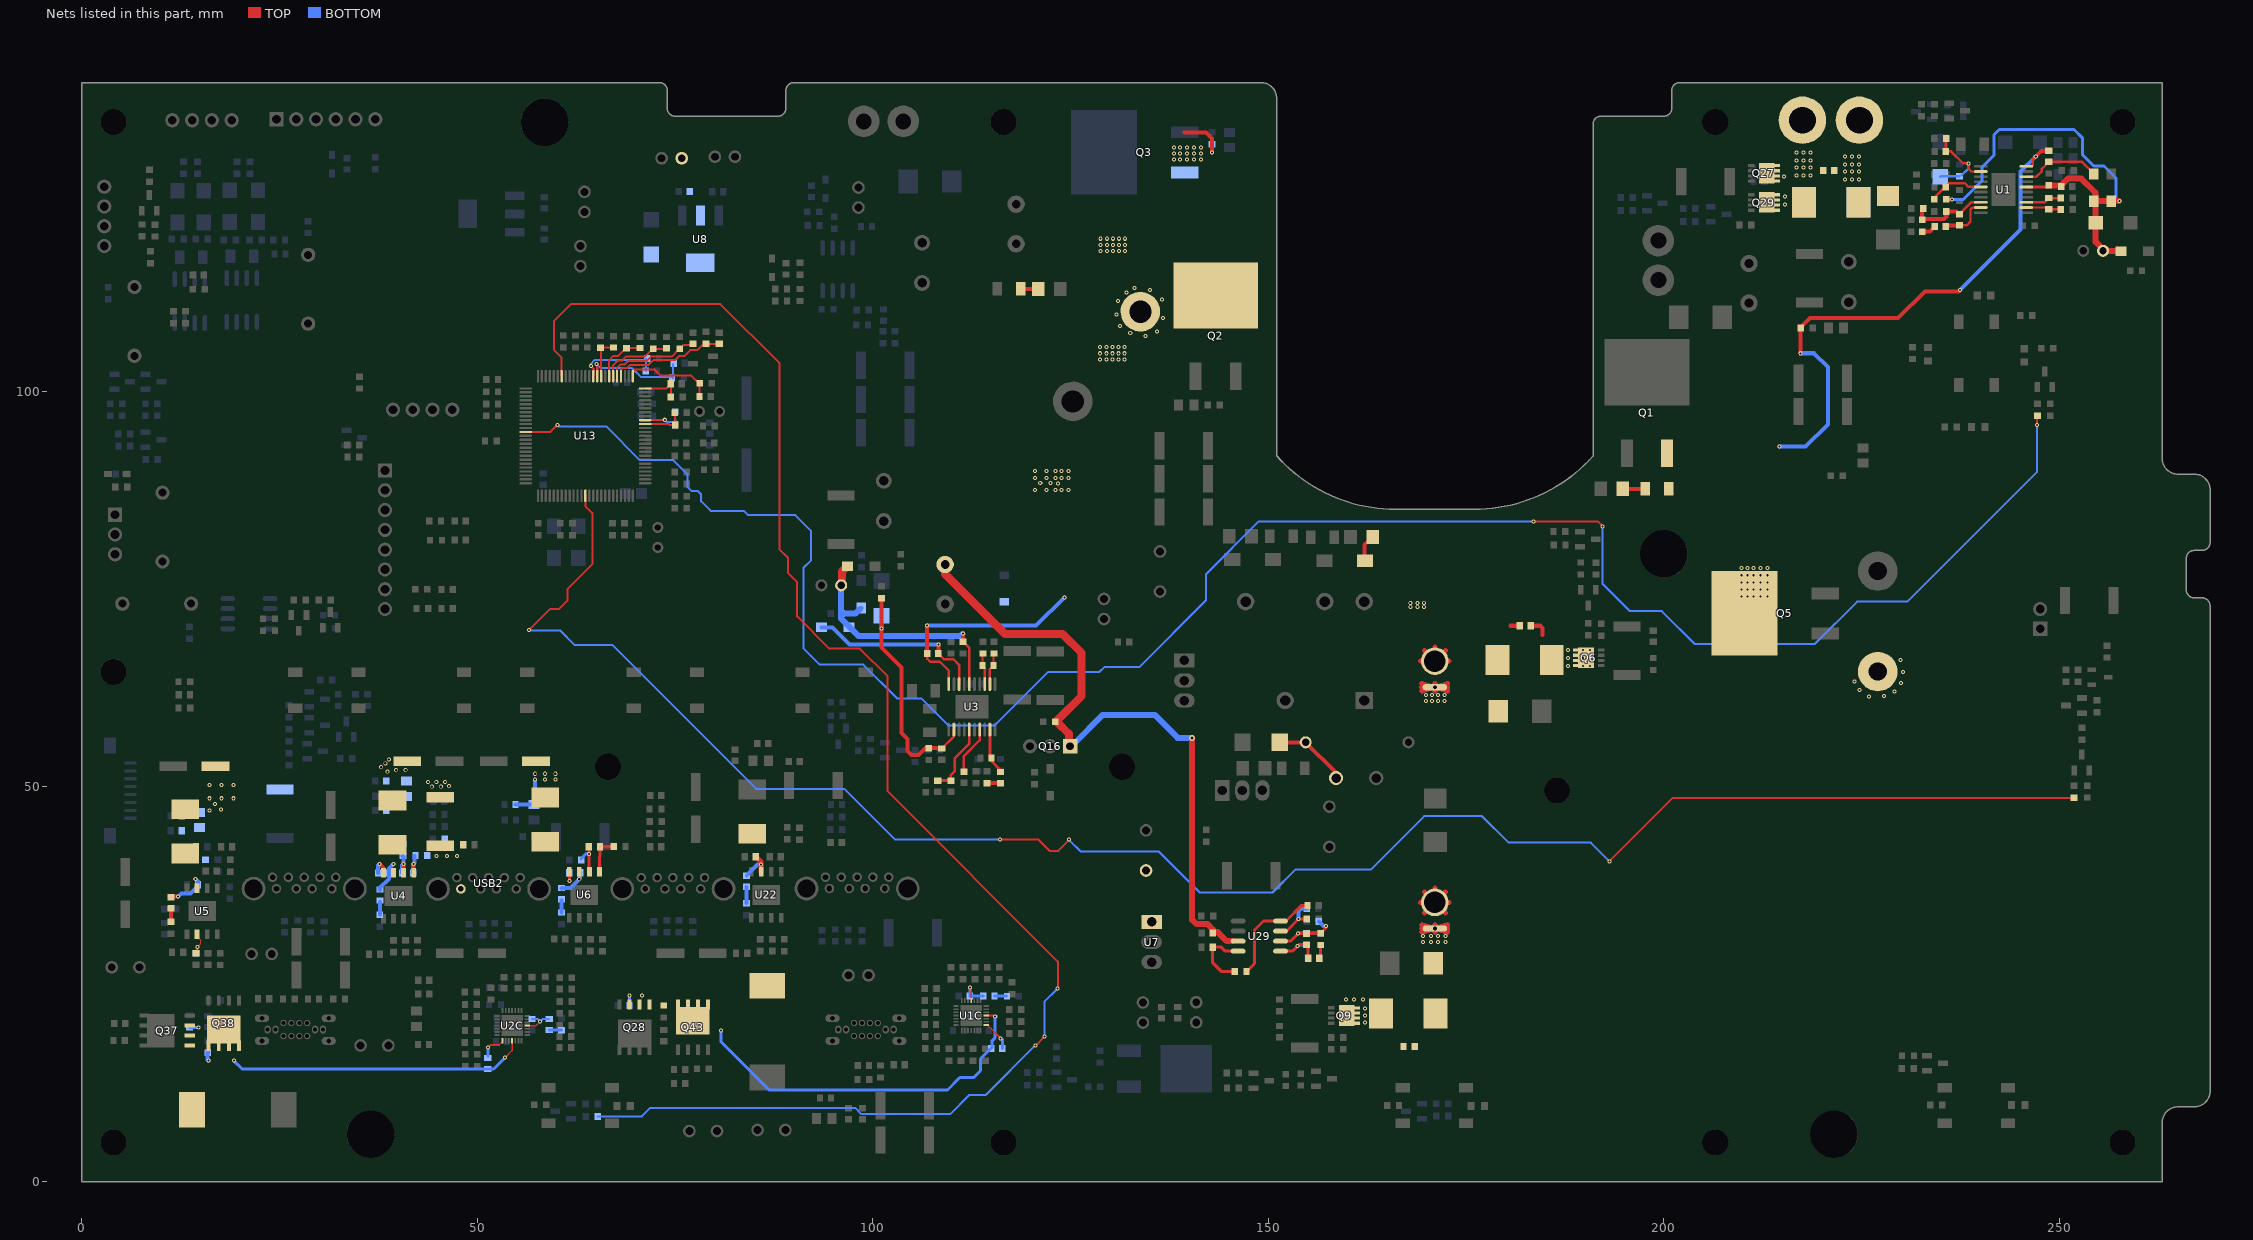
[diagram p0: the nets of this part, all layers, seen from the top]
# Altium PCB MISC84402.PcbDoc (part 6 of 12)
Units mm, origin at the board's own origin, x right, y up, seen from the top; angles counter-clockwise.
Board outline 269.06 x 139 mm, 4 copper layers (TOP, GND02, PWR03, BOTTOM), stack 0.732 mm thick; 694 components, 428 nets, 1859 pads, 1384 vias.

## Via types
v1: diameter 0.508, hole 0.254, TOP to BOTTOM, tented both sides, 1015 vias
v2: diameter 0.508, hole 0.254, TOP to BOTTOM, 243 vias
v3: diameter 0.508, hole 0.305, TOP to BOTTOM, 60 vias
v4: diameter 0.61, hole 0.305, TOP to BOTTOM, 55 vias
v5: diameter 0.61, hole 0.305, TOP to BOTTOM, tented both sides, 8 vias
v6: diameter 0.762, hole 0.381, TOP to BOTTOM, 2 vias
v7: diameter 0.762, hole 0.381, TOP to BOTTOM, tented both sides, 1 vias

## Nets (pads, with @x,y where several pads share a name; then routed paths per layer and width w, separated by ;. In a path a pad name is that pad's centre, name@x,y a point inside that pad or via, vN(x,y) a via of type N, cw(c..) or ccw(c..) an arc to the next point about the centre after c; other vN are vias at no path point) (continued)
KEY-OPEN: R333.1 U13.62 | length 257.6
  TOP w0.254: U13.62@56.103,94.826 59.215,94.826 v2(60.096,95.707) ; v2(183.54,83.49) 191.694,83.49 v2@192.253,82.931 ; v2(247.193,95.707) R333.1@247.193,96.774
  BOTTOM w0.254: v2@60.274,95.529 66.269,95.529 70.536,91.262 74.772,91.262 76.53,89.504 76.53,87.884 77.038,87.376 77.826,87.376 78.283,86.919 78.283,86.055 79.477,84.861 83.693,84.861 84.252,84.303 90.195,84.303 92.202,82.296 92.202,78.613 91.211,77.622 91.211,67.462 93.269,65.405 98.781,65.405 103.048,61.138 106.121,61.138 109.525,57.734 115.392,57.734 122.149,64.491 128.651,64.491 129.261,65.1 133.68,65.1 142.113,73.533 142.113,76.835 148.793,83.515 v2@183.515,83.515 ; v2@192.227,82.804 192.227,75.667 195.72,72.174 199.758,72.174 203.937,67.996 219.05,67.996 224.434,73.381 230.784,73.381 247.193,89.789 v2(247.193,95.707)
  other v2: 192.253,82.88
KEY-USB: R335.1 U13.44 | length 203.7
  TOP w0.254: U13.44@60.653,101.876 60.653,104.193 59.69,105.156 59.69,108.864 61.824,110.998 80.721,110.998 88.163,103.556 88.163,80.01 89.281,78.892 89.281,76.962 90.424,75.819 90.424,71.501 94.488,67.437 98.346,67.437 101.854,63.929 101.854,49.403 123.393,27.864 v2@123.393,24.613 ; v2(120.574,17.247) v2(121.691,18.364)
  BOTTOM w0.254: R335.1@65.201,8.297 70.781,8.297 71.857,9.373 97.765,9.373 98.552,8.585 109.779,8.585 112.217,11.024 114.3,11.024 v2@120.548,17.272 ; v2(121.691,18.364) 121.691,22.784 123.368,24.46 v2(123.368,24.486)
LED-EN: R287.1 U13.88 | length 241.5
  TOP w0.254: v1@56.54,69.799 59.157,72.415 60.3,72.415 61.366,73.482 61.366,73.635 61.367,74.935 64.542,78.11 64.542,84.547 63.653,85.436 U13.88@63.653,86.776 ; v2(116.078,43.307) 120.879,43.307 122.326,41.859 123.444,41.859 v2@124.841,43.256 ; v2@124.803,43.294 v2(124.816,43.307) ; v1(193.116,40.513) 193.158,40.513 193.183,40.488 193.183,40.605 201.143,48.565 R287.1@251.892,48.565
  BOTTOM w0.254: v1(56.515,69.799) v1@56.54,69.799 ; v1@56.54,69.774 56.591,69.723 60.452,69.723 62.255,67.92 67.031,67.92 85.242,49.708 96.368,49.708 102.768,43.307 v2(116.078,43.307) ; v2(124.816,43.307) v2@124.828,43.294 ; v2@124.841,43.307 124.841,43.231 126.289,41.783 136.119,41.783 141.3,36.601 150.52,36.601 153.416,39.497 162.941,39.497 169.689,46.245 177.012,46.245 180.366,42.891 190.78,42.891 193.116,40.554 v1(193.116,40.513)
MPPT-TEMP_TC: C127.2 R257.2 U13.16 | length 5.4
  TOP w0.254: U13.16@71.203,95.826 74.194,95.826 74.297,95.723 C127.2@75.002,95.723 75.018,95.723 75.018,96.42 74.965,96.473 R257.2@74.965,97.247
NETC1_1: C1.1 D2.2 R6.1 R12.2 U1.2 | length 11.8
  TOP w0.305: R12.2@235.703,131.927 235.65,131.874 C1.1@235.65,130.302 236.323,130.302 237.847,128.778 v1(238.506,128.778) 238.506,128.119 238.874,127.751 U1.2@240.078,127.751
  BOTTOM w0.305: D2.2@234.95,127.086 235,127.136 R6.1@237.363,127.136 ; R6.1@237.642,127.305 237.668,127.305 238.506,128.143 v1(238.506,128.778)
NetC3_1: C3.1 R273.2 | length 1.5
  TOP w0.508: R273.2@11.261,32.901 C3.1@11.261,34.408
NetC3_2: C3.2 C145.1 L3.1 U5.3 | length 4.9
  TOP w0.508: C3.2@11.244,36.073 v2(12.162,36.073)
  BOTTOM w0.508: v2(12.162,36.073) 12.563,36.474 13.741,36.474 C145.1@14.554,37.287 ; v1(14.377,38.319) 14.696,38 C145.1@14.696,37.43 ; C145.1@14.605,37.465 C145.1@14.661,37.409
NETC5_1: C5.1 R282.1 U13.26 | length 11.2
  TOP w0.254: U13.26@69.653,101.876 69.653,102.444 69.926,102.718 72.39,102.718 73.152,101.956 77.038,101.956 R282.1@77.953,101.041 ; C5.1@78.081,99.314 R282.1@78.081,100.837
NetC7_1: C7.1 R277.2 | length 1.6
  BOTTOM w0.508: R277.2@37.659,33.79 C7.1@37.659,35.366
NetC7_2: C7.2 C58.1 L5.1 U4.3 | length 3.9
  BOTTOM w0.508: C7.2@37.651,36.886 37.651,37.143 38.837,38.329 C58.1@38.837,38.913 ; C58.1@38.826,39.081 38.826,39.653 v1(39.396,40.224)
NetC8_1: C8.1 R278.2 | length 1.5
  BOTTOM w0.508: R278.2@60.621,34.07 C8.1@60.621,35.602
NetC8_2: C8.2 C66.1 L9.1 U6.3 | length 3.8
  BOTTOM w0.381: C66.1@63.02,39.014 C66.1@63.02,39.195
  BOTTOM w0.508: C8.2@60.613,37.114 C8.2@60.757,37.114 ; C8.2@60.757,37.16 61.747,37.16 62.967,38.379 C66.1@62.967,39.116
  other v3: 62.865,38.278
NETC10_1: C10.1 L2.1 Q1.3 Q5.2 R206.2 R253.1 U1.20 | length 69.1
  TOP w0.305: U1.20@245.824,128.401 246.511,128.401 246.634,128.524 246.634,129.286 v1(247.02,129.672)
  TOP w0.508: v1(217.297,104.775) 217.306,104.784 R253.1@217.306,107.95 217.306,108.035 218.491,109.22 229.616,109.22 232.994,112.598 237.326,112.598 237.472,112.744 v1(237.465,112.751) ; v1(247.02,129.672) 247.715,130.367 C10.1@248.666,130.367
  BOTTOM w0.508: v1(214.63,92.964) 217.932,92.964 220.726,95.758 220.726,103.048 218.999,104.775 v1(217.297,104.775) ; v1(237.465,112.751) 245.11,120.396 245.11,127.762 v1(247.02,129.672)
  other v1: 209.804,74.041 210.566,74.041 211.328,74.041 212.217,74.041 213.106,74.041 209.804,74.93 210.566,74.93 211.328,74.93 212.217,74.93 213.106,74.93 209.804,75.819 210.566,75.819 211.328,75.819 212.217,75.819 213.106,75.819 209.804,76.708 210.566,76.708 211.328,76.708 212.217,76.708 213.106,76.708 209.804,77.597 210.566,77.597 211.328,77.597 212.217,77.597 213.106,77.597
  other v2: 225.933,61.392 227.813,61.468 229.159,62.027 224.714,62.179 229.972,63.094 224.13,63.271 230.226,64.491 229.921,66.015
NETC10_2: C10.2 D21.1 U1.18 | length 10.1
  TOP w0.305: U1.18@245.824,127.101 247.108,127.101 247.802,127.795 247.802,128.103 C10.2@248.666,128.967 252.879,128.967 D21.1@254.381,127.465
NETC11_2: C11.2 C191.1 D1.2 D4.1 D39.1 R2.2 U3.16 | length 32.8
  TOP w0.305: R2.2@111.379,68.317 112.197,67.499 U3.16@112.197,62.944
  TOP w0.508: R2.2@111.379,68.317 v1(111.379,69.342)
  TOP w1.016: C191.1@96.114,75.54 96.114,77.181 D4.1@96.808,77.876
  BOTTOM w0.508: C191.1@95.992,75.438 C191.1@96.077,75.353 ; D39.1@98.378,72.386 D39.1@98.552,72.56 ; v1@111.303,69.342 v1(111.379,69.342)
  BOTTOM w0.762: C191.1@95.992,75.438 95.992,71.216 98.196,69.012 111.049,69.012 v1@111.303,69.266 ; C11.2@96.077,71.882 97.815,71.882 D39.1@98.349,72.415
NetC12_2: C12.2 C42.2 U3.5 | length 9
  TOP w0.305: C12.2@109.855,50.738 109.855,51.435 110.363,51.943 110.363,53.594 112.197,55.428 U3.5@112.197,57.198
  TOP w0.381: C42.2@108.204,50.738 C12.2@109.753,50.738
NETC13_1: C13.1 U3.7 | length 6.1
  TOP w0.305: C13.1@111.506,51.881 111.506,53.848 113.497,55.839 U3.7@113.497,57.198
NETC14_1: C14.1 R8.2 | length 1.5
  TOP w0.508: R8.2@114.427,50.428 C14.1@115.934,50.428
NETC14_2: C14.2 C130.1 U3.9 | length 6
  TOP w0.381: U3.9@114.797,57.198 114.797,53.402 C14.2@116.307,51.892
  TOP w0.508: C14.2@116.129,51.83 C14.2@116.129,51.867
NETC15_1: C15.1 D3.2 R9.1 R223.2 U3.2 | length 30.3
  TOP w0.305: R223.2@107.061,54.855 R223.2@107.114,54.802 ; C15.1@108.659,54.855 C15.1@108.712,54.802 110.247,56.337 U3.2@110.247,57.198
  TOP w0.508: R9.1@101.092,73.796 v1(101.092,69.977) 101.092,67.564 103.632,65.024 103.632,56.769 104.394,56.007 104.394,54.483 104.902,53.975 105.791,53.975 106.671,54.855 R223.2@107.061,54.855 107.721,54.855 C15.1@108.659,54.855
  BOTTOM w0.508: v1(101.092,69.977) D3.2@101.092,71.596
NetC16_1: C16.1 R25.2 U3.12 | length 4.1
  TOP w0.305: U3.12@114.797,62.944 114.797,64.821 C16.1@115.254,65.278 115.254,66.749 R25.2@115.316,66.811
NetC16_2: C16.2 R22.2 U3.13 | length 4
  TOP w0.305: R22.2@113.919,66.811 113.854,66.746 C16.2@113.854,65.278 114.147,64.985 U3.13@114.147,62.944
NetC17_1: C17.1 R279.2 | length 2
  BOTTOM w0.508: R279.2@84.039,35.29 C17.1@84.039,37.316
NetC17_2: C17.2 C151.1 L10.1 U22.3 | length 4.7
  TOP w0.508: C151.1@85.181,41.113 C151.1@85.321,40.972
  TOP w0.635: C151.1@85.344,40.996 85.878,40.462 U22.3@85.878,39.195
  BOTTOM w0.381: C17.2@84.049,38.684 C17.2@84.049,38.735 ; C17.2@84.052,38.738 C17.2@84.239,38.925
  BOTTOM w0.508: C17.2@84.226,38.938 85.42,40.131 v2(85.878,40.131)
NetC18_1: C18.1 C20.1 U1.9 | length 6.2
  TOP w0.305: C18.1@237.363,120.966 238.314,120.966 238.771,121.423 238.771,122.936 239.036,123.201 U1.9@240.078,123.201
  TOP w0.508: C20.1@235.65,120.904 C18.1@237.301,120.904
NetC18_2: C18.2 R34.2 R248.1 R306.1 U1.8 | length 10.4
  TOP w0.305: C18.2@237.298,122.366 C18.2@237.363,122.366 238.848,123.851 U1.8@240.078,123.851
  TOP w0.508: R34.2@232.782,123.063 232.664,122.945 R248.1@232.664,121.657 232.742,121.735 235.426,121.735 235.703,122.013 R306.1@235.703,122.682 236.982,122.682 C18.2@237.298,122.366
NETC19_1: C19.1 C22.1 U1C.25 | length 4.5
  TOP w0.203: v1(112.294,24.603) 112.294,24.222 112.421,24.095 112.421,23.8 112.421,23.393 U1C.25@112.421,22.954
  BOTTOM w0.381: v1@112.291,24.605 v1(112.294,24.603) C22.1@112.294,23.419 ; C22.1@112.38,23.51 C19.1@113.967,23.51
NETC19_2: C19.2 R119.1 | length 1.5
  BOTTOM w0.381: C19.2@115.367,23.51 R119.1@116.9,23.51
NETC20_2: C20.2 R248.2 | length 1.9
  TOP w0.508: R248.2@232.664,120.151 233.624,120.151 C20.2@234.25,120.777 ; C20.2@234.187,120.84 C20.2@234.25,120.904
NetC21_2: C21.2 R354.1 U13.31 | length 9
  TOP w0.254: U13.31@67.153,101.876 67.153,103.246 67.767,103.861 68.301,103.861 68.834,104.394 71.196,104.394 72.111,105.308 C21.2@73.914,105.308
NetC24_1: C24.1 R49.2 U1.12 | length 4.4
  TOP w0.305: U1.12@245.824,123.201 248.463,123.201 C24.1@248.666,122.998 R49.2@250.128,122.998
NetC24_2: C24.2 R27.2 U1.13 | length 4.7
  TOP w0.305: U1.13@245.824,123.851 248.119,123.851 C24.2@248.666,124.398 R27.2@250.19,124.398 250.243,124.398 R27.2@250.317,124.324
NetC25_2: C25.2 R198.1 | length 2.2
  TOP w0.508: R198.1@118.7,112.903 119.25,112.903 C25.2@120.901,112.903
NETC26_1: C26.1 R86.1 U13.29 | length 14.5
  TOP w0.254: U13.29@68.153,101.876 68.153,102.722 68.327,102.896 68.452,102.896 68.452,102.93 68.82,102.93 68.853,102.896 68.911,102.896 69.317,103.302 71.628,103.302 72.238,103.911 74.981,103.911 75.489,104.419 76.149,104.419 76.886,105.156 77.8,105.156 78.613,105.969 C26.1@80.442,105.969
NETC27_2: C27.2 C190.1 D15.1 D21.2 D23.1 D52.1 R274.2 R357.1 U1.16 | length 72.2
  TOP w0.381: R357.1@235.686,124.241 v2(236.439,124.241) ; U1.16@245.824,125.801 248.474,125.801 R274.2@248.666,125.993 250.116,125.993 250.15,125.959 C27.2@250.252,125.857 ; C27.2@250.419,126.136 251.13,126.848 251.155,126.873 252.857,126.873 254.381,125.349 254.381,125.247 D21.2@254.381,123.995 D21.2@254.508,123.995 ; D21.2@254.584,123.995 D21.2@254.508,123.995 ; C190.1@255.524,117.729 254.602,118.651 254.602,118.855 D52.1@254.602,121.285 254.584,121.302 254.508,121.379 D21.2@254.508,123.995 ; v2@257.523,124.003 v2(257.581,124.003)
  TOP w0.762: R274.2@248.666,125.959 250.15,125.959 250.19,125.959 250.744,126.512 250.744,126.517 251.041,126.815 251.046,126.815 251.079,126.848 251.13,126.848 252.781,126.848 254.381,125.247 254.584,125.044 D21.2@254.584,123.995 ; v2@257.523,123.995 D23.1@256.54,123.995 D21.2@254.584,123.995 ; D15.1@257.819,117.694 255.762,117.694 254.602,118.855 254.584,118.872 254.584,121.302 D21.2@254.584,123.995
  BOTTOM w0.381: v2(236.439,124.241) 236.449,124.231 237.896,124.231 240.233,126.568 240.233,128.295 241.732,129.794 241.732,132.385 242.418,133.071 251.866,133.071 252.911,132.026 252.911,131.845 252.959,131.845 252.959,129.845 254.356,128.448 255.651,128.448 257.175,126.924 257.175,124.409 v2(257.581,124.003)
NETC33_1: C33.1 L1.1 Q2.2 Q3.3 R260.1 U3.20 | length 34.6
  TOP w0.305: C33.1@106.869,66.802 106.869,66.153 107.236,65.786 108.458,65.786 109.597,64.647 U3.20@109.597,62.944
  TOP w0.508: C33.1@106.869,66.802 v1(106.869,70.358) ; 139.422,132.715 142.113,132.715 142.875,131.953 v1(142.875,130.175)
  BOTTOM w0.508: v1(106.869,70.358) 120.65,70.358 v1@124.206,73.914 ; v1(142.875,130.175) R260.1@142.875,131.2
  other v1: 124.217,73.914 120.523,87.503 121.92,87.503 123.063,87.503 123.825,87.503 124.714,87.503 123.419,88.316 121.158,88.367 122.479,88.367 120.523,89.027 121.92,89.027 123.063,89.027 123.825,89.027 124.714,89.027 120.523,89.916 121.92,89.916 123.063,89.916 123.825,89.916 124.714,89.916 128.729,104.013 129.54,104.013 130.302,104.013 131.064,104.013 131.826,104.013 128.729,104.775 129.54,104.775 130.302,104.775 131.064,104.775 131.826,104.775 128.729,105.537 129.54,105.537 130.302,105.537 131.064,105.537 131.826,105.537 128.807,117.729 129.618,117.729 130.38,117.729 131.142,117.729 131.904,117.729 128.807,118.491 129.618,118.491 130.38,118.491 131.142,118.491 131.904,118.491 128.807,119.253 129.618,119.253 130.38,119.253 131.142,119.253 131.904,119.253 138.049,129.286 138.811,129.286 139.7,129.286 140.589,129.286 141.478,129.286 138.049,130.048 138.811,130.048 139.7,130.048 140.589,130.048 141.478,130.048 138.049,130.81 138.811,130.81 139.7,130.81 140.589,130.81 141.478,130.81
  other v2: 134.442,106.985 132.537,107.315 135.915,107.544 131.267,108.204 136.703,109.22 130.785,109.652 130.988,111.379 136.525,111.582 132.055,112.446 135.026,112.801 133.045,113.005
NETC33_2: C33.2 D1.1 U3.18 | length 22.4
  TOP w0.305: C33.2@108.269,66.802 108.983,66.088 110.188,66.088 110.897,65.379 U3.18@110.897,62.944
  TOP w0.508: C33.2@108.269,66.802 v1(108.269,67.945)
  BOTTOM w0.508: D1.1@93.515,70.104 94.869,70.104 97.028,67.945 v1(108.269,67.945)
NetC34_2: C34.2 R317.1 U13.30 | length 11.5
  TOP w0.254: U13.30@67.653,101.876 67.653,102.933 68.097,103.378 68.631,103.378 69.037,103.784 71.374,103.784 71.933,104.343 74.549,104.343 R317.1@75.463,105.258 ; R317.1@75.574,105.36 75.616,105.36 76.048,105.791 C34.2@77.064,105.791
NetC35_2: C35.2 R280.2 U13.25 | length 4.8
  TOP w0.254: U13.25@71.203,100.326 73.91,100.326 74.447,100.863 74.447,99.543 R280.2@74.422,99.517
NetC36_2: C36.2 R206.1 | length 2.8
  TOP w0.508: C36.2@194.804,87.63 R206.1@197.64,87.63
NetC37_1: C37.1 R357.2 U1.5 | length 7
  TOP w0.305: R357.2@234.213,124.308 234.213,124.46 236.042,126.289 238.049,126.289 238.537,125.801 U1.5@240.078,125.801
NETC40_2: C40.2 C171.1 D18.1 Q16.1 R148.2 U29.7 | length 84.1
  TOP w0.381: U29.7@145.466,30.445 U29.7@146.172,30.445
  TOP w0.762: Q16.1@124.714,55.093 Q16.1@124.714,55.448 ; v7(140.361,56.159) 140.361,33.146 140.919,32.588 142.316,32.588 143.002,31.902 143.002,31.598 143.612,31.598 144.755,30.455 U29.7@145.466,30.455
  TOP w1.016: C171.1@109.133,78.065 109.133,76.871 116.713,69.291 123.977,69.291 126.365,66.904 126.365,61.417 123.342,58.395 123.342,58.09 124.765,56.667 Q16.1@124.765,55.448
  BOTTOM w0.508: v7@140.31,56.159 v7(140.361,56.159)
  BOTTOM w0.762: Q16.1@125.019,55.27 Q16.1@125.019,55.423 ; Q16.1@125.425,55.423 129.057,59.055 135.636,59.055 138.532,56.159 v7@140.31,56.159
NETC41_1: C41.1 D6.1 D7.1 J4.2 Q27.5 Q27.6 Q27.7 Q27.8 Q27.9 Q29.5 Q29.6 Q29.7 Q29.8 Q29.9
  other v1: 215.327,123.581 215.327,124.597 215.2,127.137 216.789,127.254 217.678,127.254 218.567,127.254 216.789,128.27 217.678,128.27 218.567,128.27 216.789,129.159 217.678,129.159 218.567,129.159 216.789,130.175 217.678,130.175 218.567,130.175
NETC41_2: C41.2 D6.2 D7.2 F2.2 J4.1
  other v1: 222.885,126.746 223.774,126.746 224.663,126.746 222.885,127.762 223.774,127.762 224.663,127.762 222.885,128.651 223.774,128.651 224.663,128.651 222.885,129.667 223.774,129.667 224.663,129.667
NETC45_1: C45.1 R117.2 U29.8 | length 8.6
  TOP w0.381: R117.2@145.728,26.594 144.102,26.594 142.966,27.73 142.966,29.683 144.044,29.683 144.552,29.175 U29.8@146.172,29.175
NETC47_1: C47.1 D8.1 J2.2 Q9.5 Q9.6 Q9.7 Q9.8 Q9.9 | length 21.5
  TOP w0.635: 169.448,31.597 J2.2@171.049,32.048 ; 169.448,32.048 J2.2@171.049,32.048 ; 169.448,32.5 J2.2@171.049,32.048 ; 171.049,31.597 J2.2@171.049,32.048 ; 171.049,32.5 J2.2@171.049,32.048 ; 172.651,31.597 J2.2@171.049,32.048 ; 172.651,32.048 J2.2@171.049,32.048 ; 172.651,32.5 J2.2@171.049,32.048
  BOTTOM w0.635: 169.448,31.597 J2.2@171.049,32.048 ; 169.448,32.048 J2.2@171.049,32.048 ; 169.448,32.5 J2.2@171.049,32.048 ; 171.049,31.597 J2.2@171.049,32.048 ; 171.049,32.5 J2.2@171.049,32.048 ; 172.651,31.597 J2.2@171.049,32.048 ; 172.651,32.048 J2.2@171.049,32.048 ; 172.651,32.5 J2.2@171.049,32.048
  other v1: 162.205,20.158 162.205,21.047 162.205,21.936 159.792,23.079 160.808,23.079 161.951,23.079 169.571,30.318 170.587,30.318 171.476,30.318 172.365,30.318 169.571,31.08 170.587,31.08 171.476,31.08 172.365,31.08
NETC47_2: C47.2 D8.2 F3.2 J2.1 | length 12.9
  TOP w0.635: 169.248,35.35 J2.1@171.049,35.35 ; 169.725,34.026 J2.1@171.049,35.35 ; 169.725,36.675 J2.1@171.049,35.35 ; 171.049,37.152 J2.1@171.049,35.35 ; 172.374,34.026 J2.1@171.049,35.35 ; 172.374,36.675 J2.1@171.049,35.35 ; 172.851,35.35 J2.1@171.049,35.35
NETC48_1: C48.1 D9.1 J3.2 Q6.5 Q6.6 Q6.7 Q6.8 Q6.9 | length 24.5
  TOP w0.254: Q6.9@190.653,66.767 v1(190.653,67.275)
  TOP w0.508: C48.1@183.162,70.323 184.43,70.323 184.684,70.069 184.684,69.18
  TOP w0.635: 169.448,62.097 J3.2@171.049,62.548 ; 169.448,62.548 J3.2@171.049,62.548 ; 169.448,63 J3.2@171.049,62.548 ; 171.049,62.097 J3.2@171.049,62.548 ; 171.049,63 J3.2@171.049,62.548 ; 172.651,62.097 J3.2@171.049,62.548 ; 172.651,62.548 J3.2@171.049,62.548 ; 172.651,63 J3.2@171.049,62.548
  BOTTOM w0.635: 169.448,62.097 J3.2@171.049,62.548 ; 169.448,62.548 J3.2@171.049,62.548 ; 169.448,63 J3.2@171.049,62.548 ; 171.049,62.097 J3.2@171.049,62.548 ; 171.049,63 J3.2@171.049,62.548 ; 172.651,62.097 J3.2@171.049,62.548 ; 172.651,62.548 J3.2@171.049,62.548 ; 172.651,63 J3.2@171.049,62.548
  other v1: 169.952,60.798 170.714,60.798 171.476,60.798 172.238,60.798 169.952,61.56 170.714,61.56 171.476,61.56 172.238,61.56 187.859,65.243 189.764,65.243 190.653,65.243 187.859,66.259 189.764,66.259 190.653,66.259 187.859,67.275 189.764,67.275
NETC48_2: C48.2 D9.2 F4.2 J3.1 | length 10.3
  TOP w0.508: 180.62,70.323 C48.2@181.763,70.323
  TOP w0.635: 169.248,65.85 J3.1@171.049,65.85 ; 169.725,67.175 J3.1@171.049,65.85 ; 171.049,67.652 J3.1@171.049,65.85 ; 172.374,67.175 J3.1@171.049,65.85 ; 172.851,65.85 J3.1@171.049,65.85
NETC49_2: C49.2 R28.1 R76.1 R343.1 USB2.1
  other v1: 44.857,41.24 46.127,41.24 47.397,41.24
NETC50_1: C50.1 R343.2 U4.1 | length 3.4
  TOP w0.508: U4.1@41.936,39.068 v1(41.936,40.224)
  BOTTOM w0.508: C50.1@41.874,39.081 41.874,40.161 v1(41.936,40.224) 42.072,40.36 R343.2@42.072,41.24
NETC50_2: C50.2 R342.2 U4.2 | length 3.5
  TOP w0.508: U4.2@40.666,39.068 v1(40.666,40.224)
  BOTTOM w0.508: C50.2@40.474,39.081 40.474,40.032 v1(40.666,40.224) 40.666,41.104 R342.2@40.53,41.24
NetC52_1: C52.1 R284.1 U13.35 | length 13.3
  TOP w0.254: v2(65.049,103.429) 65.151,103.327 U13.35@65.151,102.489
  BOTTOM w0.254: v2(65.049,103.429) 65.583,102.895 69.545,102.895 70.663,101.778 R284.1@74.66,101.778 ; R284.1@74.727,101.752 74.701,101.778 R284.1@74.66,101.778 ; R284.1@74.753,101.685 R284.1@74.66,101.778 ; R284.1@74.755,101.603 C52.1@74.755,103.438
NETC57_2: C57.2 C106.2 L8.2 R28.2 R342.1
  other v3: 44.247,49.987 45.39,49.987 46.406,50.038 43.764,50.571 44.806,50.571 45.923,50.571
NETC58_2: C58.2 U4.4 | length 2.6
  TOP w0.508: v1(37.618,40.224) 38.126,39.716 U4.4@38.126,39.068
  BOTTOM w0.508: C58.2@37.426,39.081 37.426,40.032 v1(37.618,40.224)
NETC66_2: C66.2 U6.4 | length 2.3
  TOP w0.381: v1(61.621,38.065) U6.4@61.621,39.195
  BOTTOM w0.381: v1(61.621,38.065) C66.2@61.621,39.195
NETC67_1: C67.1 R134.1 | length 1.7
  TOP w0.381: C67.1@156.428,28.286 156.617,28.475 R134.1@156.617,29.954
NETC67_2: C67.2 C81.1 R168.2 U29.1 | length 6.6
  TOP w0.381: U29.1@151.537,29.175 153.061,29.175 v1(153.696,29.81) 153.885,29.999 C81.1@154.839,29.999 155.028,29.81 C67.2@155.028,28.286
  BOTTOM w0.381: v1(153.696,29.81) 153.84,29.954 R168.2@154.839,29.954
NETC68_1: C68.1 R341.2 U6.1 | length 4.9
  TOP w0.381: U6.1@65.431,39.195 65.431,41.113 65.496,41.178 C68.1@65.496,42.383 R341.2@67.218,42.383
NETC68_2: C68.2 R340.2 U6.2 | length 4.5
  TOP w0.381: U6.2@64.084,39.272 U6.2@64.096,39.26 ; U6.2@64.096,39.206 U6.2@64.096,39.26 ; C68.2@64.096,42.383 v1(64.096,41.494) U6.2@64.096,39.26 ; U6.2@64.161,39.195 U6.2@64.096,39.26
  BOTTOM w0.381: R340.2@63.084,40.853 63.735,41.504 v1@64.059,41.504
NETC70_1: C70.1 R258.2 U29.3 | length 6.1
  TOP w0.381: U29.3@151.537,31.715 152.299,31.715 v1(153.823,33.239) R258.2@154.848,33.239
  BOTTOM w0.508: v1(153.823,33.239) 153.823,34.232 154.186,34.595 C70.1@154.872,34.595
NetC73_1: C73.1 R285.2 U13.36 | length 10.5
  TOP w0.254: v2(64.338,103.149) 64.653,102.835 U13.36@64.653,101.876
  BOTTOM w0.254: v2@64.313,103.2 64.313,103.411 64.839,103.937 71.095,103.937 71.29,104.131 C73.1@71.29,102.532
NetC74_1: C74.1 R286.2 U13.17 | length 5.2
  TOP w0.254: U13.17@71.203,96.326 v2@73.694,96.326
  BOTTOM w0.254: v2(73.685,96.368) v2@73.685,96.469 ; v2@73.711,96.317 73.965,96.063 74.524,96.063 74.663,96.063 C74.1@74.984,95.742 ; C74.1@74.955,96.037 R286.2@74.955,97.13
NetC75_1: C75.1 C157.1 D13.1 U7.1 | length 2.5
  TOP w0.508: 162.128,79.375 162.128,80.565 C157.1@163.088,81.525
  other v3: 167.97,72.72 168.859,72.72 169.672,72.72 167.945,73.203 168.859,73.203 169.672,73.228
NETC77_1: C77.1 C102.2 L3.2 L4.1
  other v1: 16.129,46.99 17.551,47.066 16.815,47.803 16.129,48.514 17.653,48.514 19.177,48.514 16.129,50.165 17.653,50.165 19.177,50.165
NETC81_2: C81.2 R134.2 R149.2 R168.1 R190.1 U29.2 | length 10.4
  TOP w0.381: U29.2@151.537,30.445 152.804,30.445 v1(153.758,31.398) C81.2@154.839,31.399 155.728,31.398 155.79,31.46 R134.2@156.617,31.461 157.259,32.103 v1(157.259,32.36)
  BOTTOM w0.381: v1(153.758,31.398) 153.82,31.46 R168.1@154.839,31.461 R149.2@156.617,31.461
  BOTTOM w0.508: R168.1@154.839,31.461 R168.1@154.872,31.494 ; R190.1@156.378,32.944 156.963,32.36
NetC82_1: C82.1 U1C.15 | length 3.8
  TOP w0.203: U1C.15@114.478,19.837 v1(116.154,18.161)
  BOTTOM w0.381: v1@116.154,18.186 116.356,17.984 C82.1@116.356,16.881
NETC82_2: C82.2 L6.1 Q28.1 Q28.2 Q28.3 Q43.5 Q43.6 Q43.7 Q43.8 R126.2 R174.2 U1C.18 | length 47.8
  TOP w0.203: U1C.18@114.328,21.047 115.342,21.047 v1(115.469,20.92)
  BOTTOM w0.381: R126.2@69.232,22.317 v1(69.232,23.578) ; v1(80.798,19.142) 80.798,19.075 80.797,17.729 86.893,11.633 109.423,11.633 110.998,13.208 112.751,13.208 113.614,14.072 113.614,15.57 115.037,16.993 115.037,17.805 115.468,18.237 115.468,20.879 v1(115.469,20.92)
  other v1: 70.827,23.587
NetC85_2: C85.2 C94.1 D14.2 U8.2 U8.4
NetC86_1: C86.1 U2C.15 | length 3.3
  TOP w0.203: v1(51.308,16.993) 51.638,17.323 52.73,17.323 53.182,17.774 U2C.15@53.182,17.869
  BOTTOM w0.381: C86.1@51.308,15.954 51.308,16.916 v1@51.333,16.942
NETC86_2: C86.2 L7.1 Q37.1 Q37.2 Q37.3 Q38.5 Q38.6 Q38.7 Q38.8 R212.2 R226.2 U2C.18 | length 40.1
  TOP w0.203: v1@53.543,15.773 54.382,16.612 U2C.18@54.382,17.869
  TOP w0.254: v1(53.493,15.713) v1@53.548,15.768
  BOTTOM w0.381: R212.2@13.615,19.54 v1(14.758,19.54) ; v1(19.203,15.332) 20.26,14.275 52.055,14.275 v1(53.493,15.713)
  BOTTOM w0.508: R226.2@15.927,16.383 R226.2@15.901,16.356 15.901,15.459 v1(16.028,15.332)
NETC89_1: C89.1 R117.1 U29.4 | length 13.7
  TOP w0.381: R117.1@147.234,26.594 148.242,27.602 148.242,31.849 149.378,32.985 U29.4@151.537,32.985 152.22,32.985 154.211,34.976 C89.1@154.954,34.976
NetC92_2: C92.2 R243.2 U5.6 | length 3
  TOP w0.127: R243.2@14.453,29.159 v2@14.453,29.54 ; U5.6@14.558,31.346 14.558,31.026 15.021,30.562 15.021,30.109 14.656,29.743 v2(14.63,29.718)
  BOTTOM w0.127: C92.2@14.63,29.083 14.63,29.413 v2(14.63,29.718)
NETC95_1: C95.1 C114.2 L9.2 L11.1 | length 5.5
  BOTTOM w0.508: C114.2@54.819,47.71 57.09,47.71 57.302,47.923 v1@57.302,50.851
  other v1: 57.303,50.892 58.573,50.892 59.843,50.892
  other v3: 57.302,51.613 58.547,51.613 59.842,51.613
NETC98_1: C98.1 D20.1 R16.1 | length 9.4
  TOP w0.508: D20.1@151.432,55.591 R16.1@154.712,55.591 158.556,51.747 C98.1@158.556,51.071
NetC99_2: C99.2 R355.1 U13.32 | length 6
  TOP w0.254: U13.32@66.65,102.413 66.65,103.911 67.183,104.445 67.779,104.445 68.764,105.43 C99.2@70.552,105.43
NetC100_2: C100.2 R356.1 U13.34 | length 5
  TOP w0.254: R356.1@65.541,105.487 C100.2@67.056,105.487 ; U13.34@65.653,101.876 R356.1@65.653,105.315
NetC101_2: C101.2 C144.2 L4.2 R31.2 R345.1
NetC103_2: C103.2 C104.1 U2C.25 | length 4.3
  TOP w0.203: U2C.25@56.289,19.777 57.445,19.777 v1@57.963,20.295
  BOTTOM w0.254: C103.2@56.922,20.603 57.619,20.603 v1(57.938,20.285) 58.257,20.603 C104.1@59.081,20.604
NETC104_2: C104.2 R88.1 | length 1.6
  BOTTOM w0.381: C104.2@59.081,19.204 60.629,19.204 R88.1@60.639,19.194
NetC105_2: C105.2 C122.1 L5.2 L8.1
  other v3: 38.633,51.867 39.726,52.07 40.919,52.07 37.821,52.451 38.354,52.934 38.811,53.416